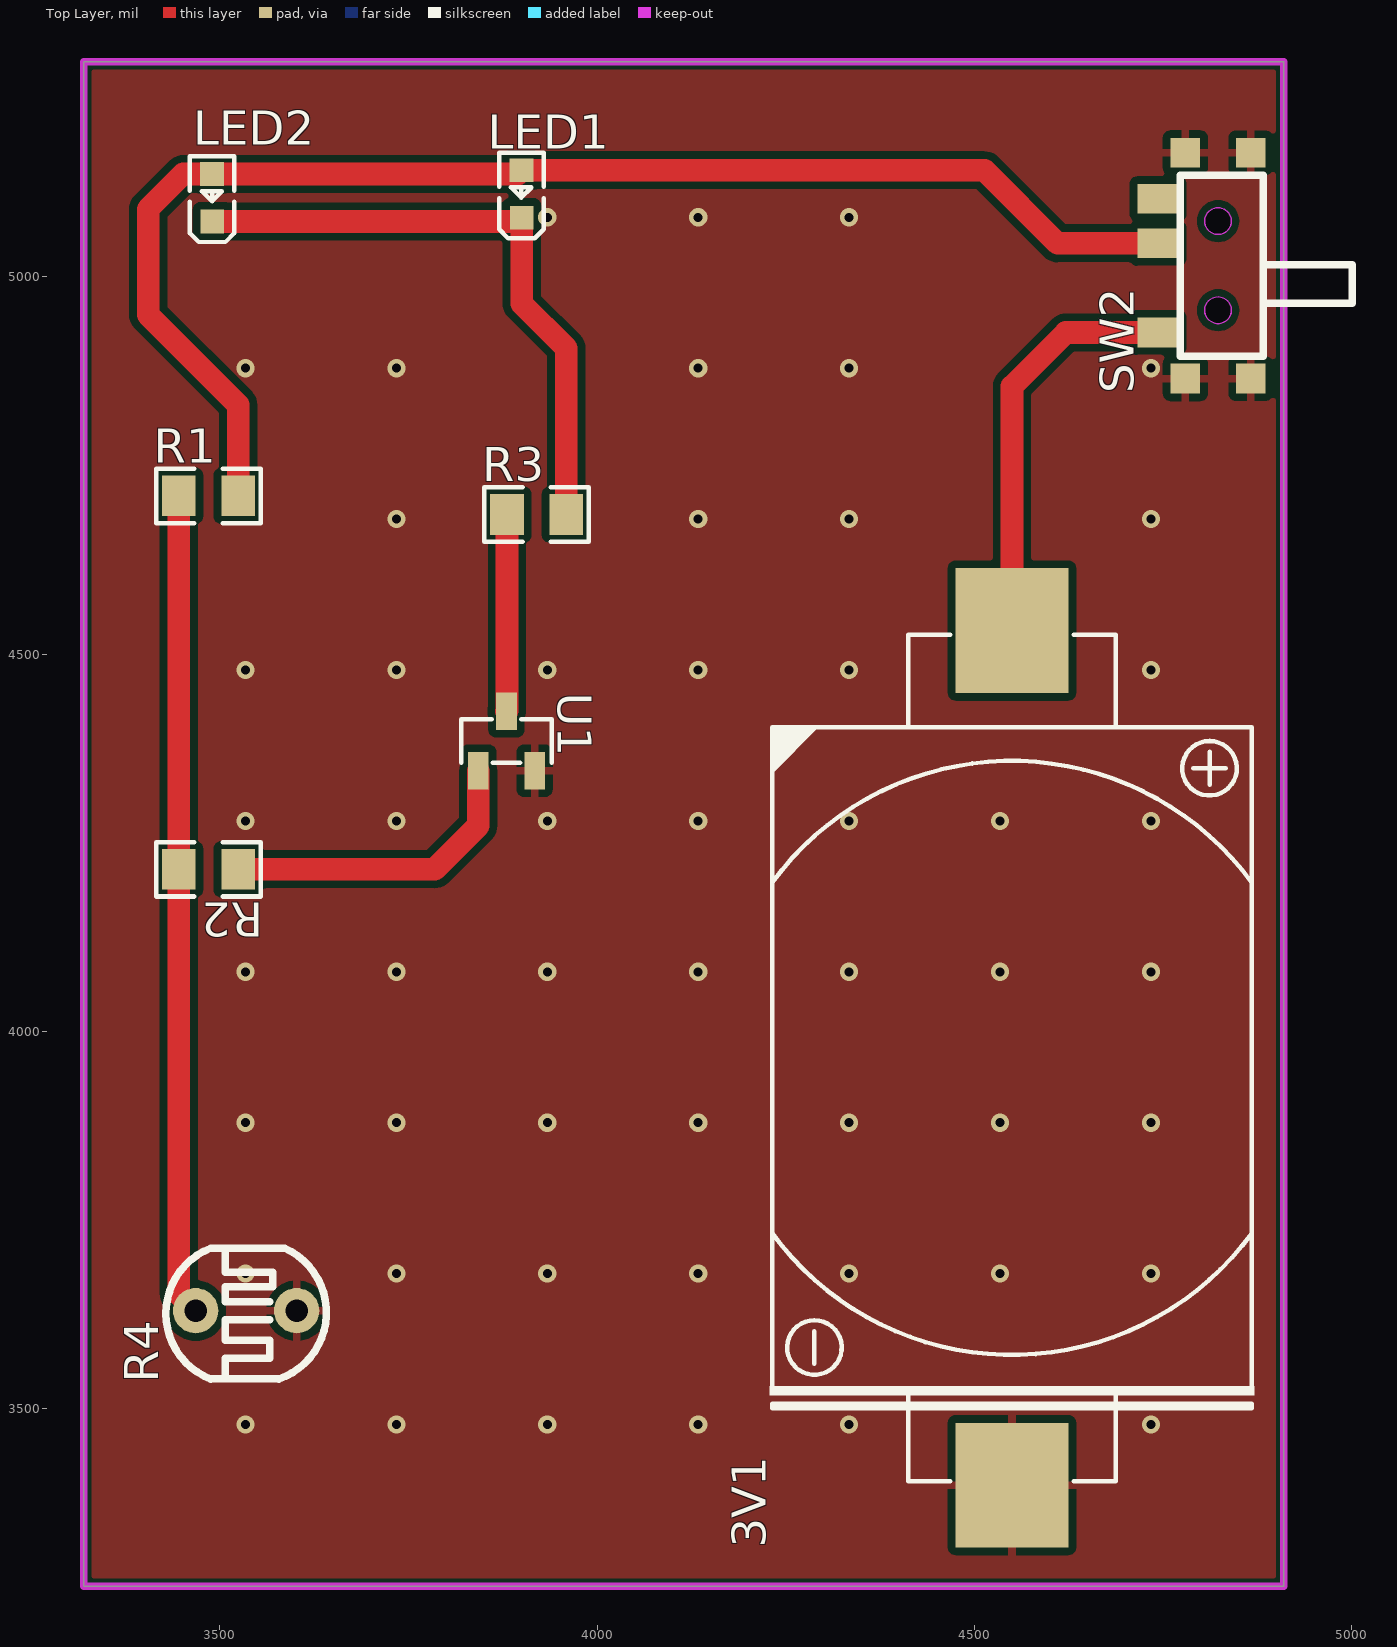
[diagram p0: Top Layer view]
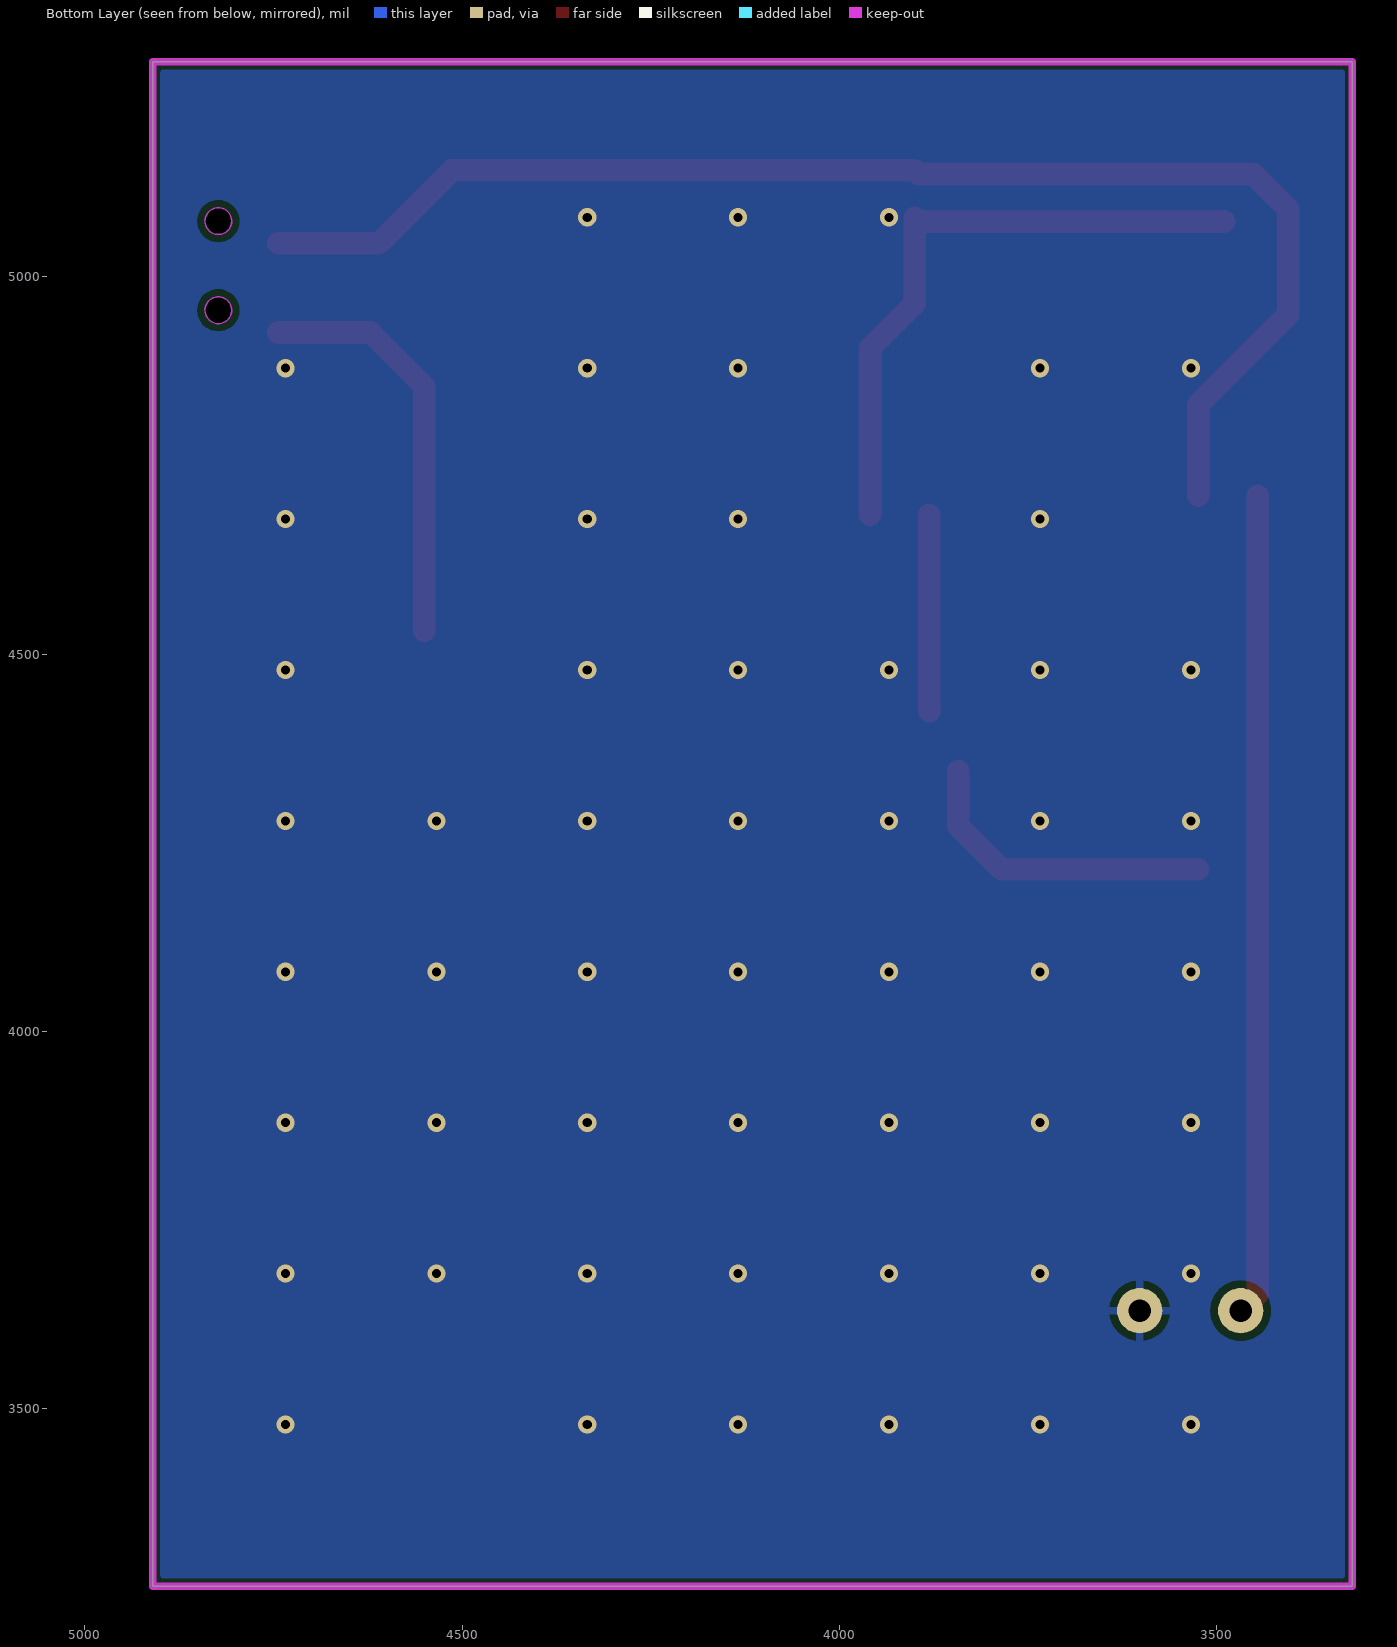
[diagram p1: Bottom Layer view, seen from below]
# Altium PCB MISC51059.pcbdoc
Units mil, origin at the board's own origin, x right, y up, seen from the top; angles counter-clockwise.
Board outline 1590 x 2020 mil, 2 copper layers (Top Layer, Bottom Layer), stack 62.206 mil thick; 9 components, 7 nets, 24 pads, 52 vias.

## Layer stack, top to bottom
Top Solder Mask Layer: solder mask 0.394, Dk 3.3
Top Layer: signal copper 1.379
Dielectric1: surface 59.449, FR4, Dk 4.5
Bottom Layer: signal copper 1.378
Bottom Solder Mask Layer: solder mask 0.394, Dk 3.3

## Board outline
3320,5285 3320,3265 4910,3265 4910,5285

## Design rules (kind name [scope] priority, off if disabled: settings)
BoardOutlineClearance copperThickness2oz_1 [All] p2 off: genericclearance=7.99 ignorepadtopadclearanceinfootprint=FALSE except(0: Arc-SplitContinuation Track-SplitContinuation SMDPad-SplitContinuation THPad-SplitContinuation Via-SplitContinuation Fill-SplitContinuation Region-SplitContinuation Poly-SplitContinuation Text-SplitContinuation Hole-SplitContinuation; 5.98: Arc-CutoutEdge SMDPad-CutoutEdge THPad-CutoutEdge Via-CutoutEdge Fill-CutoutEdge Region-CutoutEdge Text-CutoutEdge; 6.93: Hole-OutlineEdge Hole-CutoutEdge; 10: Poly-OutlineEdge Poly-CutoutEdge; 11.81: Arc-OutlineEdge Track-OutlineEdge SMDPad-OutlineEdge THPad-OutlineEdge Via-OutlineEdge Fill-OutlineEdge Region-OutlineEdge Text-OutlineEdge Track-CutoutEdge)
BoardOutlineClearance copperThickness1oz_1 [All] p4: genericclearance=4.02 ignorepadtopadclearanceinfootprint=FALSE except(0: Arc-SplitContinuation Track-SplitContinuation SMDPad-SplitContinuation THPad-SplitContinuation Via-SplitContinuation Fill-SplitContinuation Region-SplitContinuation Poly-SplitContinuation Text-SplitContinuation Hole-SplitContinuation; 6: SMDPad-CutoutEdge THPad-CutoutEdge Via-CutoutEdge Fill-CutoutEdge Region-CutoutEdge Text-CutoutEdge; 6.93: Hole-OutlineEdge Hole-CutoutEdge; 10: Poly-OutlineEdge Poly-CutoutEdge; 11.8: Arc-OutlineEdge Track-OutlineEdge SMDPad-OutlineEdge THPad-OutlineEdge Via-OutlineEdge Fill-OutlineEdge Region-OutlineEdge Text-OutlineEdge; 11.81: Arc-CutoutEdge Track-CutoutEdge)
Clearance copperThickness2oz [All] p1 off: gap=7.99 ignorepadtopadclearanceinfootprint=FALSE except(5.98: SMDPad-Track SMDPad-SMDPad THPad-Track SMDPad-THPad THPad-THPad Track-Via SMDPad-Via THPad-Via Via-Via Fill-Track Region-Track Fill-SMDPad Region-SMDPad Fill-THPad Region-THPad Fill-Via Region-Via Fill-Fill Fill-Region Region-Region Arc-Track Arc-SMDPad Arc-THPad Arc-Via Fill-Arc Region-Arc Arc-Arc Text-Track SMDPad-Text Text-THPad Text-Via Fill-Text Region-Text Arc-Text Text-Text; 6.93: Hole-Track Hole-SMDPad Hole-THPad Hole-Via Fill-Hole Region-Hole Hole-Arc Hole-Text; 10: Poly-Track Poly-SMDPad Poly-THPad Poly-Via Poly-Fill Poly-Region Poly-Poly Poly-Arc Poly-Text Poly-Hole)
Clearance copperThickness1oz [All] p3: gap=4.02 ignorepadtopadclearanceinfootprint=FALSE except(5.98: SMDPad-Track SMDPad-SMDPad THPad-Track SMDPad-THPad THPad-THPad Track-Via SMDPad-Via THPad-Via Via-Via Fill-Track Region-Track Fill-SMDPad Region-SMDPad Fill-THPad Region-THPad Fill-Via Region-Via Fill-Fill Fill-Region Region-Region; 6: Arc-Track Arc-SMDPad Arc-THPad Arc-Via Fill-Arc Region-Arc Arc-Arc Text-Track SMDPad-Text Text-THPad Text-Via Fill-Text Region-Text Arc-Text Text-Text; 6.93: Hole-Track Hole-SMDPad Hole-THPad Hole-Via Fill-Hole Region-Hole Hole-Arc Hole-Text; 10: Poly-Track Poly-SMDPad Poly-THPad Poly-Via Poly-Fill Poly-Region Poly-Poly Poly-Arc Poly-Text Poly-Hole)
Creepage creepage [All] p1: checkdistance=0 ignoreinternallayers=TRUE applytopolygonpour=TRUE
DiffPairsRouting differentialPair [All] p1: maxlimit=6 minlimit=6 mostfreqgap=6 toplayer_minwidth=5 toplayer_prefwidth=10 toplayer_maxwidth=100 toplayer_mingap=6 toplayer_prefgap=6 toplayer_maxgap=6 bottomlayer_minwidth=5 bottomlayer_prefwidth=10 bottomlayer_maxwidth=100 bottomlayer_mingap=6 bottomlayer_prefgap=6 bottomlayer_maxgap=6 maxuncoupledlength=10
HoleToHoleClearance otherClearance [All] p1: gap=11.81 allowstackedmicrovias=TRUE
Length netLength [All] p1: minlimit=0 maxlimit=0
MatchedLengths netLengthTolerance [All] p1: tolerance=1000
PasteMaskExpansion pasteMaskExpansion [All] p1: expansion=0
PlaneConnect innerPlane [All] p1: planeconnectstyle=Relief reliefexpansion=20 reliefentries=4 reliefconductorwidth=10 reliefairgap=10
PolygonConnect copperRegion [(InNet('GND'))] p1: connectstyle=Relief reliefconductorwidth=10 reliefentries=4 polygonreliefangle="90 Angle" airgapwidth=10 via.connectstyle=Relief via.reliefconductorwidth=10 via.reliefentries=4 via.polygonreliefangle="90 Angle" via.airgapwidth=10
RoutingVias viaSize [All] p1: holewidth=12.01 width=24.02 viastyle="Through Hole" minholewidth=11.81 minwidth=19.68 maxholewidth=248.03 maxwidth=393.7
SolderMaskExpansion solderMaskExpansion [IsVia] p1: expansion=-1000 istentingtop=TRUE
SolderMaskExpansion solderMaskExpansion [All] p2: expansion=2 istentingtop=FALSE
Width copperThickness2oz_2 [All] p1 off: maxlimit=100 minlimit=8 preferedwidth=10
Width copperThickness1oz_2 [All] p2: maxlimit=100 minlimit=5 preferedwidth=10

## Components (designator, comment, footprint, x,y, rotation, side; value= is the part's Value field where it differs from the comment)
3V1 "" BAT-TH_CR2032-BS-6-1 4550,3965 r90 top
LED1 "NCD0603W1" LED0603-RD 3900,5110 r90 top
LED2 "NCD0603W1" LED0603-RD 3490,5105 r90 top
R1 "4.7kΩ" R0805 3485,4710 r0 top
R2 "1K" R0805 3485,4215 r180 top
R3 "100" R0805 3920,4685 r0 top
R4 "GL3516（5-10K）" RES-TH_L5.1-W4.3-P3.40-D0.5 3535,3630 r90 top
SW2 "SK-3296S-01-L1" SW-SMD_3P-P1.50_L2.7-W6.6 4805,5015 r90 top
U1 "S9013" SOT-23-3_L2.9-W1.3-P1.90-LS2.4-BR 3880,4385 r270 top

## Footprints (in the part's own frame and the unit in brackets; to place one, negate y for a bottom-side part, rotate by r counter-clockwise, add the part's x,y. Pads: shape width x height; smd on the part's side, far side on the other; paste and mask are expansions set on the pad)
BAT-TH_CR2032-BS-6-1 [mm]
  rect 4.2x3.8 smd: 1(14.385,0) 2(-14.385,0)
  silkscreen extent -14.25,-8.15 14.25,8.15
LED0603-RD [mm]
  rect 0.8x0.8 smd: 1(-0.799,-0.003) 2(0.799,0.003)
  silkscreen extent -1.49,-0.75 1.39,0.76
R0805 [mm]
  rect 1.133x1.377 smd paste-100 mask+0.051: 1(-1,0) 2(1,0)
  silkscreen extent -1.76,-0.92 1.76,0.92
RES-TH_L5.1-W4.3-P3.40-D0.5 [mil]
  round 60 hole 30: 1(0,66.93) 2(0,-66.93)
  silkscreen extent -91,-106 83,106
SOT-23-3_L2.9-W1.3-P1.90-LS2.4-BR [mm]
  rect 1.25x0.7 smd: 1(1,-0.95) 2(1,0.95) 3(-1,0)
  silkscreen extent -0.73,-1.53 0.73,1.53
SW-SMD_3P-P1.50_L2.7-W6.6 [mm]
  rect 1x1 smd: 0(-3.8,-1.559) 0(-3.8,0.641) 0(3.8,-1.559) 0(3.8,0.641)
  rect 1x1.4 smd: 1(-2.25,1.559) 2(0.75,1.559) 3(2.25,1.559)
  Board Outline Layer circle w0.003: c-1.5,-0.459 r0.45
  Board Outline Layer circle w0.003: c1.5,-0.459 r0.45
  Board Outline Layer region: -1.5,-0.909 -1.695,-0.864 -1.852,-0.74 -1.939,-0.559 -1.939,-0.359 -1.852,-0.178 -1.695,-0.054 -1.5,-0.009 -1.5,-0.009 -1.305,-0.054 -1.148,-0.178 -1.061,-0.359 -1.061,-0.559 -1.148,-0.74 -1.305,-0.864 -1.5,-0.909
  Board Outline Layer region: -1.5,-0.909 -1.593,-0.899 -1.683,-0.87 -1.764,-0.823 -1.834,-0.76 -1.89,-0.684 -1.928,-0.598 -1.947,-0.506 -1.947,-0.412 -1.928,-0.32 -1.89,-0.234 -1.834,-0.158 -1.764,-0.095 -1.683,-0.048 -1.593,-0.019 -1.5,-0.009 -1.406,-0.019 -1.317,-0.048 -1.235,-0.095 -1.165,-0.158 -1.11,-0.234 -1.072,-0.32 -1.052,-0.412 -1.052,-0.506 -1.072,-0.598 -1.11,-0.684 -1.165,-0.76 -1.235,-0.823 -1.317,-0.87 -1.406,-0.899
  Board Outline Layer region: 1.5,-0.909 1.305,-0.864 1.148,-0.74 1.061,-0.559 1.061,-0.359 1.148,-0.178 1.305,-0.054 1.5,-0.009 1.5,-0.009 1.695,-0.054 1.852,-0.178 1.939,-0.359 1.939,-0.559 1.852,-0.74 1.695,-0.864 1.5,-0.909
  Board Outline Layer region: 1.5,-0.909 1.407,-0.899 1.317,-0.87 1.236,-0.823 1.166,-0.76 1.11,-0.684 1.072,-0.598 1.053,-0.506 1.053,-0.412 1.072,-0.32 1.11,-0.234 1.166,-0.158 1.236,-0.095 1.317,-0.048 1.407,-0.019 1.5,-0.009 1.594,-0.019 1.683,-0.048 1.765,-0.095 1.835,-0.158 1.89,-0.234 1.928,-0.32 1.948,-0.412 1.948,-0.506 1.928,-0.598 1.89,-0.684 1.835,-0.76 1.765,-0.823 1.683,-0.87 1.594,-0.899
  Multi-Layer board cut-out: -1.5,-0.909 -1.695,-0.864 -1.852,-0.74 -1.939,-0.559 -1.939,-0.359 -1.852,-0.178 -1.695,-0.054 -1.5,-0.009 -1.5,-0.009 -1.305,-0.054 -1.148,-0.178 -1.061,-0.359 -1.061,-0.559 -1.148,-0.74 -1.305,-0.864 -1.5,-0.909
  Multi-Layer board cut-out: 1.5,-0.909 1.305,-0.864 1.148,-0.74 1.061,-0.559 1.061,-0.359 1.148,-0.178 1.305,-0.054 1.5,-0.009 1.5,-0.009 1.695,-0.054 1.852,-0.178 1.939,-0.359 1.939,-0.559 1.852,-0.74 1.695,-0.864 1.5,-0.909
  silkscreen extent -3.05,-4.98 3.05,0.81

## Via types
v1: diameter 24.02, hole 12, Top Layer to Bottom Layer, 52 vias

## Nets (pads, with @x,y where several pads share a name; then routed paths per layer and width w, separated by ;. In a path a pad name is that pad's centre, name@x,y a point inside that pad or via, vN(x,y) a via of type N, cw(c..) or ccw(c..) an arc to the next point about the centre after c; other vN are vias at no path point)
$1N1: LED1.2 LED2.2 R1.2 SW2.2 | length 1829.5
  Top Layer w30: R1.2 3524.37,4830.63 3405,4950 3405,5090 3451.47,5136.48 LED2.2 3894.86,5136.48 LED1.2 4513.52,5141.48 4610.47,5044.53 SW2.2
$1N2: 3V1.1 SW2.1 | length 546.9
  Top Layer w30: 3V1.1 4550,4855 4621.42,4926.42 SW2.1
$1N8: LED1.1 LED2.1 R3.2 | length 830.1
  Top Layer w30: LED2.1 3895.14,5073.52 LED1.1 3900.14,4964.86 3959.37,4905.63 R3.2
$1N9: R1.1 R2.2 R4.1 | length 1089.3
  Top Layer w30: R1.1 R2.2 3445.63,3652.44 R4.1
$1N10: R3.1 U1.3 | length 260.9
  Top Layer w30: U1.3 3880.63,4425 R3.1
$1N11: R2.1 U1.1 | length 415.1
  Top Layer w30: R2.1 3785,4215 3842.6,4272.6 U1.1
GND: 3V1.2 R4.2 SW2.0 U1.2
  other v1: 3534.1,3479.1 3734.1,3479.1 3934.1,3479.1 4134.1,3479.1 4334.1,3479.1 4734.1,3479.1 3534.1,3679.1 3734.1,3679.1 3934.1,3679.1 4134.1,3679.1 4334.1,3679.1 4534.1,3679.1 4734.1,3679.1 3534.1,3879.1 3734.1,3879.1 3934.1,3879.1 4134.1,3879.1 4334.1,3879.1 4534.1,3879.1 4734.1,3879.1 3534.1,4079.1 3734.1,4079.1 3934.1,4079.1 4134.1,4079.1 4334.1,4079.1 4534.1,4079.1 4734.1,4079.1 3534.1,4279.1 3734.1,4279.1 3934.1,4279.1 4134.1,4279.1 4334.1,4279.1 4534.1,4279.1 4734.1,4279.1 3534.1,4479.1 3734.1,4479.1 3934.1,4479.1 4134.1,4479.1 4334.1,4479.1 4734.1,4479.1 3734.1,4679.1 4134.1,4679.1 4334.1,4679.1 4734.1,4679.1 3534.1,4879.1 3734.1,4879.1 4134.1,4879.1 4334.1,4879.1 4734.1,4879.1 3934.1,5079.1 4134.1,5079.1 4334.1,5079.1
pads on no net: SW2.3

## Polygon pours and split planes (outlines as drawn)
GND on Top Layer (solid, remove dead copper, pour order 0): 3020,5355 3020,3130 5135,3130 5135,5355
GND on Bottom Layer (solid, remove dead copper, pour order 2): 3000,5550 3000,3000 5310,3000 5310,5550

## Keep-outs
Board Outline Layer:
  the board outline again, w10